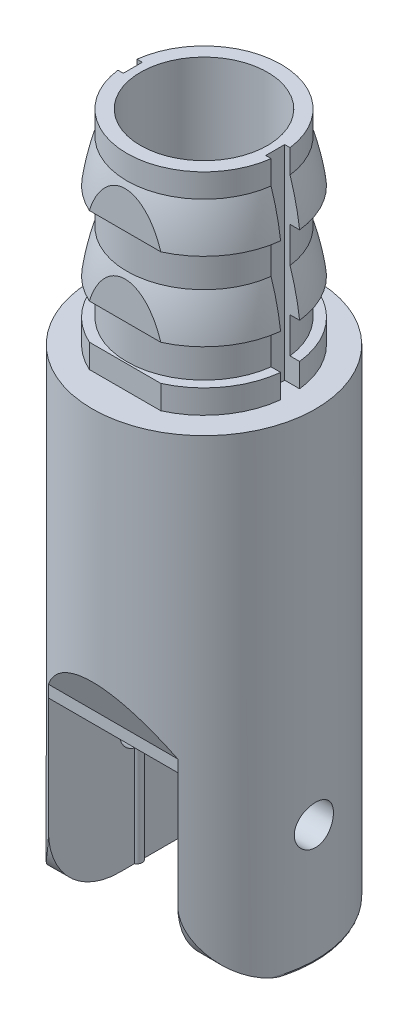
from build123d import *

# Parameters (mm, degrees)
SKETCH_3_R          = 2.675
CUT_EXTRUDE_1_DEPTH = 19.5
SKETCH_4_W          = 5.45
SKETCH_4_H          = 7.768663762
CUT_EXTRUDE_2_DEPTH = 7.86
CUT_EXTRUDE_4_REACH = 31.557
SKETCH_6_W          = 1.34037146
SKETCH_6_H          = 0.8
SKETCH_6_W_2        = 4
SKETCH_6_H_2        = 0.810357856
FILLET_8_R          = 0.1
SKETCH_7_R          = 1
CUT_EXTRUDE_5_DEPTH = 10
EXTRUDE_1_DEPTH     = 7.86
SKETCH_5_R          = 0.825
CUT_EXTRUDE_3_DEPTH = 5


with BuildPart() as part:
    # 草图1 → 旋转1 (revolve)
    with BuildSketch(Plane.XY, mode=Mode.PRIVATE) as revolve_1_sk:
        with BuildLine():
            Line((0, 0), (-4.7, 0))
            Line((-4.7, 0), (-4.7, 20.2))
            Line((-4.7, 20.2), (-3.65, 20.2))
            Line((-3.65, 20.2), (-3.65, 21.2))
            Line((-3.65, 21.2), (-3.25, 21.2))
            Line((-3.25, 21.2), (-3.25, 22.7))
            Line((-3.25, 22.7), (-3.65, 22.7))
            ThreePointArc((-3.65, 22.7), (-3.491576489, 23.60923922), (-3.25, 24.5))
            Line((-3.25, 24.5), (-3.25, 26))
            Line((-3.25, 26), (-3.65, 26))
            ThreePointArc((-3.65, 26), (-3.491576489, 26.90923922), (-3.25, 27.8))
            Line((-3.25, 27.8), (-3.25, 28.8))
            Line((-3.25, 28.8), (0, 28.8))
            Line((0, 28.8), (0, 0))
        make_face()
    revolve(revolve_1_sk.sketch.rotate(Axis((0, 40.719898965, 0), (0, -1, 0)), 270), axis=Axis((0, 40.719898965, 0), (0, -1, 0)))

    # 草图3 → 切除-拉伸1 (cut)
    with BuildSketch(Plane(origin=(0, 28.8, 0), x_dir=(1, 0, 0), z_dir=(0, 1, 0))):
        with Locations(Location((0, 0, 0), (0, 0, 270))):
            Circle(SKETCH_3_R)
    extrude(amount=-CUT_EXTRUDE_1_DEPTH, mode=Mode.SUBTRACT)

    # 草图4 → 切除-拉伸2 (cut)
    with BuildSketch(Plane.XZ):
        with Locations((0, 1.034331881)):
            Rectangle(SKETCH_4_W, SKETCH_4_H)
    extrude(amount=-CUT_EXTRUDE_2_DEPTH, mode=Mode.SUBTRACT)

    # 切除-拉伸4: up to this face of the body (flat: up to its plane)
    cut_extrude_4_end = Plane(part.part.faces().sort_by_distance((0, 20.2, -4.567063925))[0])
    # 草图6 → 切除-拉伸4 (cut, up to the picked face)
    with BuildSketch(Plane(origin=(0, 28.8, 0), x_dir=(1, 0, 0), z_dir=(0, 1, 0)), mode=Mode.PRIVATE) as cut_extrude_4_sk1:
        with Locations((-3.67018573, 0)):
            Rectangle(SKETCH_6_W, SKETCH_6_H)
    cut_extrude_4_tool1 = split(extrude(cut_extrude_4_sk1.sketch, amount=-CUT_EXTRUDE_4_REACH, mode=Mode.PRIVATE), bisect_by=cut_extrude_4_end, keep=Keep.BOTH, mode=Mode.PRIVATE)
    # 草图6 → 切除-拉伸4 (cut, up to the picked face)
    with BuildSketch(Plane(origin=(0, 28.8, 0), x_dir=(1, 0, 0), z_dir=(0, 1, 0)), mode=Mode.PRIVATE) as cut_extrude_4_sk2:
        with Locations((3.67018573, 0)):
            Rectangle(SKETCH_6_W, SKETCH_6_H)
    cut_extrude_4_tool2 = split(extrude(cut_extrude_4_sk2.sketch, amount=-CUT_EXTRUDE_4_REACH, mode=Mode.PRIVATE), bisect_by=cut_extrude_4_end, keep=Keep.BOTH, mode=Mode.PRIVATE)
    # 草图6 → 切除-拉伸4 (cut, up to the picked face)
    with BuildSketch(Plane(origin=(0, 28.8, 0), x_dir=(1, 0, 0), z_dir=(0, 1, 0)), mode=Mode.PRIVATE) as cut_extrude_4_sk3:
        with Locations((0, -3.730178928)):
            Rectangle(SKETCH_6_W_2, SKETCH_6_H_2)
    cut_extrude_4_tool3 = split(extrude(cut_extrude_4_sk3.sketch, amount=-CUT_EXTRUDE_4_REACH, mode=Mode.PRIVATE), bisect_by=cut_extrude_4_end, keep=Keep.BOTH, mode=Mode.PRIVATE)
    # 草图6 → 切除-拉伸4 (cut, up to the picked face)
    with BuildSketch(Plane(origin=(0, 28.8, 0), x_dir=(1, 0, 0), z_dir=(0, 1, 0)), mode=Mode.PRIVATE) as cut_extrude_4_sk4:
        with Locations((0, 3.730178928)):
            Rectangle(SKETCH_6_W_2, SKETCH_6_H_2)
    cut_extrude_4_tool4 = split(extrude(cut_extrude_4_sk4.sketch, amount=-CUT_EXTRUDE_4_REACH, mode=Mode.PRIVATE), bisect_by=cut_extrude_4_end, keep=Keep.BOTH, mode=Mode.PRIVATE)
    add(cut_extrude_4_tool1.solids().sort_by(Axis((-3.670186, 28.8, 0), (0, -1, 0)))[0], mode=Mode.SUBTRACT)
    add(cut_extrude_4_tool2.solids().sort_by(Axis((3.670186, 28.8, 0), (0, -1, 0)))[0], mode=Mode.SUBTRACT)
    add(cut_extrude_4_tool3.solids().sort_by(Axis((0, 28.8, 3.730179), (0, -1, 0)))[0], mode=Mode.SUBTRACT)
    add(cut_extrude_4_tool4.solids().sort_by(Axis((0, 28.8, -3.730179), (0, -1, 0)))[0], mode=Mode.SUBTRACT)

    # 圆角8
    fillet_8_edges = [part.edges().sort_by_distance(p)[0] for p in [
        (0, 0, -4.7),
    ]]
    fillet(fillet_8_edges, radius=FILLET_8_R)

    # 草图7 → 切除-拉伸5 (cut)
    with BuildSketch(Plane(origin=(0, 9.3, 0), x_dir=(1, 0, 0), z_dir=(0, 1, 0))):
        with Locations(Location((0, 0, 0), (0, 0, 270))):
            Circle(SKETCH_7_R)
    extrude(amount=-CUT_EXTRUDE_5_DEPTH, mode=Mode.SUBTRACT)

    # 草图8 → 凸台-拉伸1 (add)
    with BuildSketch(Plane.XZ):
        with BuildLine():
            Line((2.725, -0.2), (2.725, 0.2))
            ThreePointArc((2.725, 0.2), (2.6, 0), (2.725, -0.2))
        make_face()
        with BuildLine():
            Line((-2.725, -0.2), (-2.725, 0.2))
            ThreePointArc((-2.725, 0.2), (-2.6, 0), (-2.725, -0.2))
        make_face()
    extrude(amount=-EXTRUDE_1_DEPTH)

    # 草图5 → 切除-拉伸3 (cut, symmetric)
    with BuildSketch(Plane(origin=(0, 0, 0), x_dir=(0, 0, -1), z_dir=(1, 0, 0))):
        with Locations((0, 5.025)):
            Circle(SKETCH_5_R)
        Polygon((-4.7, 10.24), (-3.829409223, 8.36), (-3.829409223, 7.86), (-3.829409223, 3.115780314), (-4.7, 3.115780314), align=None)
        with BuildLine():
            Line((-3.829409223, 3), (-4.605698774, 3))
            Line((-4.605698774, 3), (-4.605698774, 0))
            Line((-4.605698774, 0), (-0.829409223, 0))
            ThreePointArc((-0.829409223, 0), (-2.950729567, 0.878679656), (-3.829409223, 3))
        make_face()
    extrude(amount=CUT_EXTRUDE_3_DEPTH, both=True, mode=Mode.SUBTRACT)


solid = part.part
